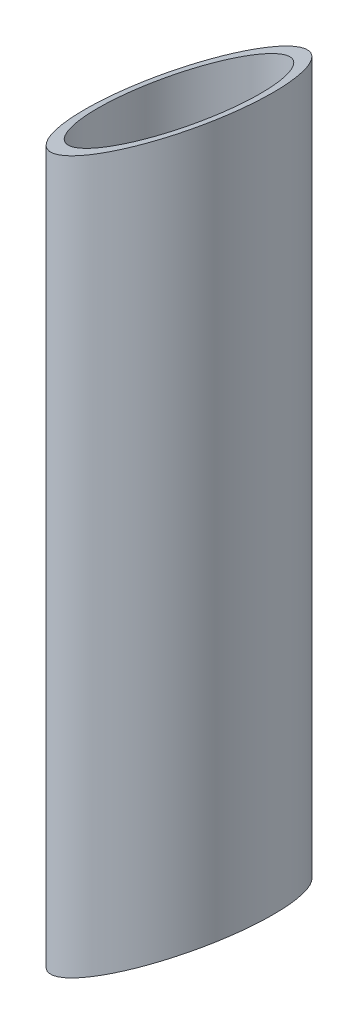
SolidWorks part; units mm, degrees
ref_plane "Front Plane" through (0, 0, 0) normal (0, 0, 1) x (1, 0, 0)
ref_plane "Top Plane" through (0, 0, 0) normal (0, 1, 0) x (1, 0, 0)
ref_plane "Right Plane" through (0, 0, 0) normal (1, 0, 0) x (0, 0, -1)
sketch "Sketch1" plane through (0, 0, 0) normal (0, 1, 0) x (1, 0, 0)
  circle A0 centre (0, 0) radius 9.5
  circle A1 centre (0, 0) radius 11
  dimension "D1" = 19
  dimension "D2" = 22
extrude "Boss-Extrude1" add sketch "Sketch1" along normal mid plane 96
sketch "Sketch2" plane through (0, 0, 0) normal (0, 0, 1) x (1, 0, 0)
  line L0 (11, 48) -> (-11, 48)
  line L1 (-11, 48) -> (-11, 35.2983)
  line L2 (-11, 35.2983) -> (11, 48)
  line L3 (11, -35.2983) -> (11, -48)
  line L4 (11, -48) -> (-11, -48)
  line L5 (-11, -48) -> (11, -35.2983)
  line L6 (9.5, 48) -> (-9.5, 48) construction
  line L7 (11, -48) -> (11, 48) construction
  line L8 (-11, 48) -> (-11, -48) construction
  line L9 (-11, -48) -> (11, -48) construction
  dimension "D1" = 30
  dimension "D2" = 30
extrude "Cut-Extrude1" cut sketch "Sketch2" against normal through all and the other way through all
